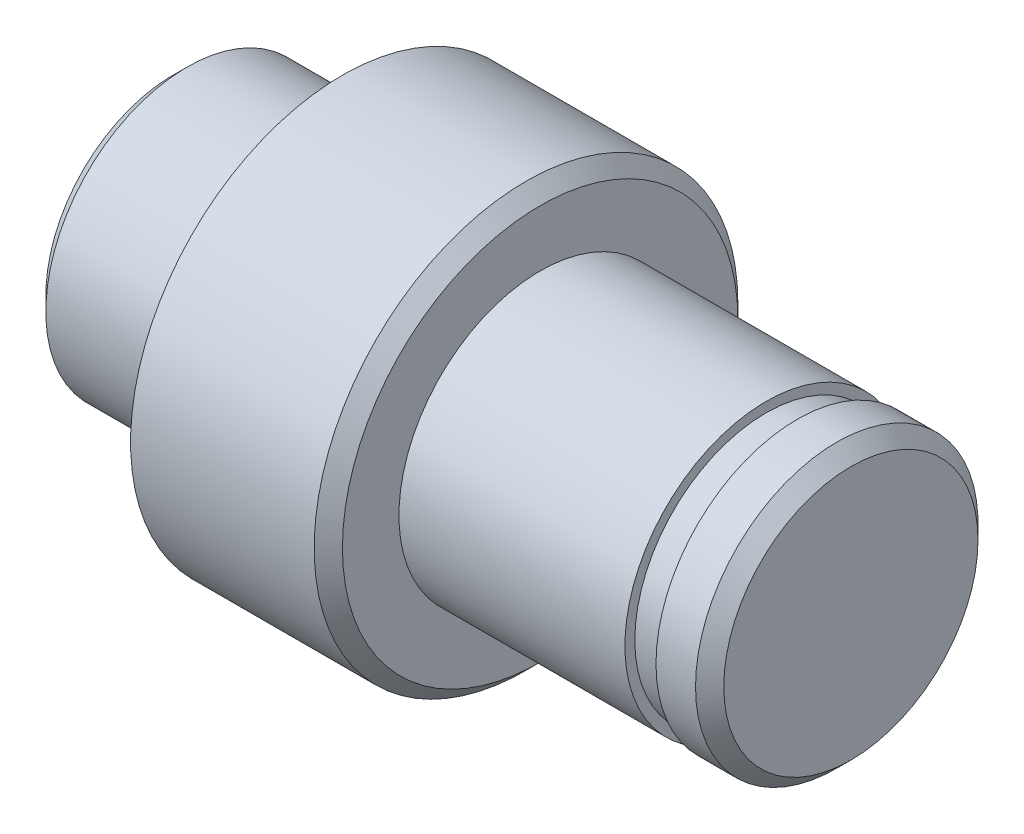
from build123d import *

# Parameters (mm, degrees)
SKETCH_1_R      = 5
EXTRUDE_1_DEPTH = 6
CHAMFER_1_SIZE  = 0.5
SKETCH_2_R      = 7.5
EXTRUDE_2_DEPTH = 7
CHAMFER_2_SIZE  = 0.5
SKETCH_3_R      = 5
EXTRUDE_3_DEPTH = 8
SKETCH_4_R      = 4.65
EXTRUDE_4_DEPTH = 1.1
SKETCH_5_R      = 5
EXTRUDE_5_DEPTH = 1.9
CHAMFER_3_SIZE  = 0.5


with BuildPart() as part:
    # 草图1 → 凸台-拉伸1 (new body)
    with BuildSketch(Plane(origin=(0, 0, 0), x_dir=(0, 0, -1), z_dir=(1, 0, 0))):
        Circle(SKETCH_1_R)
    extrude(amount=EXTRUDE_1_DEPTH)

    # 倒角1
    chamfer_1_edges = [part.edges().sort_by_distance(p)[0] for p in [
        (0, 0, 5),
    ]]
    chamfer(chamfer_1_edges, length=CHAMFER_1_SIZE)

    # 草图2 → 凸台-拉伸2 (add)
    with BuildSketch(Plane(origin=(6, 0, 0), x_dir=(0, 0, -1), z_dir=(1, 0, 0))):
        Circle(SKETCH_2_R)
    extrude(amount=EXTRUDE_2_DEPTH)

    # 倒角2
    chamfer_2_edges = [part.edges().sort_by_distance(p)[0] for p in [
        (13, 0, 7.5),
    ]]
    chamfer(chamfer_2_edges, length=CHAMFER_2_SIZE)

    # 草图3 → 凸台-拉伸3 (add)
    with BuildSketch(Plane(origin=(13, 0, 0), x_dir=(0, 0, -1), z_dir=(1, 0, 0))):
        Circle(SKETCH_3_R)
    extrude(amount=EXTRUDE_3_DEPTH)

    # 草图4 → 凸台-拉伸4 (add)
    with BuildSketch(Plane(origin=(21, 0, 0), x_dir=(0, 0, -1), z_dir=(1, 0, 0))):
        Circle(SKETCH_4_R)
    extrude(amount=EXTRUDE_4_DEPTH)

    # 草图5 → 凸台-拉伸5 (add)
    with BuildSketch(Plane(origin=(22.1, 0, 0), x_dir=(0, 0, -1), z_dir=(1, 0, 0))):
        Circle(SKETCH_5_R)
    extrude(amount=EXTRUDE_5_DEPTH)

    # 倒角3
    chamfer_3_edges = [part.edges().sort_by_distance(p)[0] for p in [
        (24, 0, 5),
    ]]
    chamfer(chamfer_3_edges, length=CHAMFER_3_SIZE)


solid = part.part
